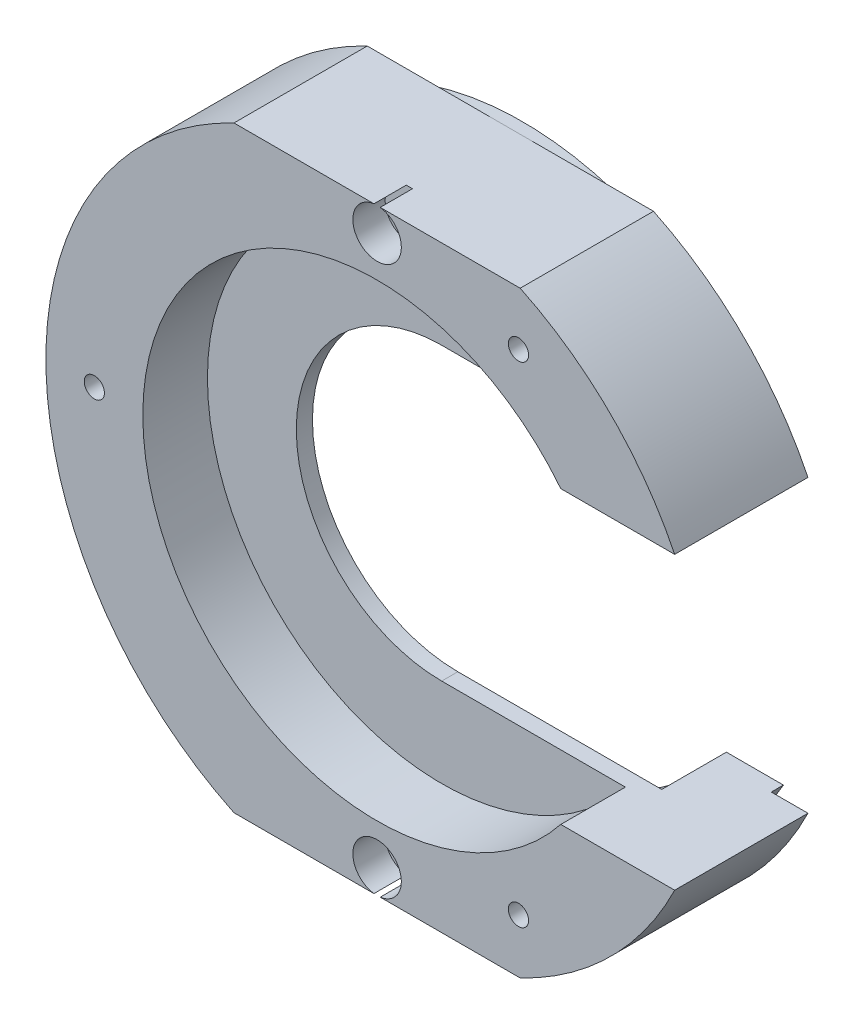
from build123d import *

# Parameters (mm, degrees)
SKETCH1_R                               = 41
BOSS_EXTRUDE1_DEPTH                     = 16.5
SKETCH2_R                               = 36.975
BOSS_EXTRUDE2_DEPTH                     = 1.5
SKETCH4_W                               = 50
SKETCH4_H                               = 6.84002239
CUT_EXTRUDE1_DEPTH                      = 61.712436947
SKETCH5_R                               = 31
CUT_EXTRUDE3_DEPTH                      = 8
SKETCH6_R                               = 29
CUT_EXTRUDE4_DEPTH                      = 8
CUT_EXTRUDE5_DEPTH                      = 57.108382841
CUT_EXTRUDE5_DEPTH_BACK                 = 57.108382841
CBORE_FOR_M3_HEX_HEAD_BOLT3_D           = 3.5
CBORE_FOR_M3_HEX_HEAD_BOLT3_CBORE_D     = 6
CBORE_FOR_M3_HEX_HEAD_BOLT3_CBORE_DEPTH = 4
M3_TAPPED_HOLE1_D                       = 2.5
CIRPATTERN1_COUNT                       = 3


with BuildPart() as part:
    # Sketch1 → Boss-Extrude1 (new body)
    with BuildSketch(Plane.XY):
        Circle(SKETCH1_R)
    extrude(amount=BOSS_EXTRUDE1_DEPTH)

    # Sketch2 → Boss-Extrude2 (add)
    with BuildSketch(Plane(origin=(0, 0, 0), x_dir=(-1, 0, 0), z_dir=(0, 0, -1))):
        Circle(SKETCH2_R)
    extrude(amount=BOSS_EXTRUDE2_DEPTH)

    # Sketch4 → Cut-Extrude1 (cut, through all)
    with BuildSketch(Plane(origin=(0, 0, -1.5), x_dir=(-1, 0, 0), z_dir=(0, 0, -1))):
        with Locations((0, 40.395011195)):
            Rectangle(SKETCH4_W, SKETCH4_H)
        with Locations((0, -40.395011195)):
            Rectangle(SKETCH4_W, SKETCH4_H)
    extrude(amount=-CUT_EXTRUDE1_DEPTH, mode=Mode.SUBTRACT)

    # Sketch5 → Cut-Extrude3 (cut)
    with BuildSketch(Plane(origin=(0, 0, -1.5), x_dir=(-1, 0, 0), z_dir=(0, 0, -1))):
        Circle(SKETCH5_R)
    extrude(amount=-CUT_EXTRUDE3_DEPTH, mode=Mode.SUBTRACT)

    # Sketch6 → Cut-Extrude4 (cut)
    with BuildSketch(Plane.XY.offset(16.5)):
        Circle(SKETCH6_R)
    extrude(amount=-CUT_EXTRUDE4_DEPTH, mode=Mode.SUBTRACT)

    # Sketch7 → Cut-Extrude5 (cut, two sides: drawn at the far end of the back side and taken through both)
    with BuildSketch(Plane.XY.offset(8.5).offset(-CUT_EXTRUDE5_DEPTH_BACK)):
        with BuildLine():
            Line((0, 18), (36.837480913, 18))
            ThreePointArc((36.837480913, 18), (41, 0), (36.837480913, -18))
            Line((36.837480913, -18), (0, -18))
            ThreePointArc((0, -18), (-18, 0), (0, 18))
        make_face()
    extrude(amount=CUT_EXTRUDE5_DEPTH + CUT_EXTRUDE5_DEPTH_BACK, mode=Mode.SUBTRACT)

    # CBORE for M3 Hex Head Bolt3 (through all)
    with Locations(Plane(origin=(0, 34, 16.5), x_dir=(1, 0, 0), z_dir=(0, 0, 1))):
        with Locations((0, 0), (0, -68)):
            CounterBoreHole(CBORE_FOR_M3_HEX_HEAD_BOLT3_D / 2, CBORE_FOR_M3_HEX_HEAD_BOLT3_CBORE_D / 2, CBORE_FOR_M3_HEX_HEAD_BOLT3_CBORE_DEPTH)

    # M3 Tapped Hole1 (through all)
    with Locations(Plane(origin=(-35, 0, 16.5), x_dir=(1, 0, 0), z_dir=(0, 0, 1))):
        with Locations((0, 0)):
            m3_tapped_hole1 = Hole(M3_TAPPED_HOLE1_D / 2)

    # CirPattern1: M3 Tapped Hole1 ×3 about axis
    cirpattern1_axis = Axis((0, 0, 0), (0, 0, 1))
    for i in range(1, CIRPATTERN1_COUNT):
        add(m3_tapped_hole1.rotate(cirpattern1_axis, i * 360 / CIRPATTERN1_COUNT), mode=Mode.SUBTRACT)


solid = part.part
